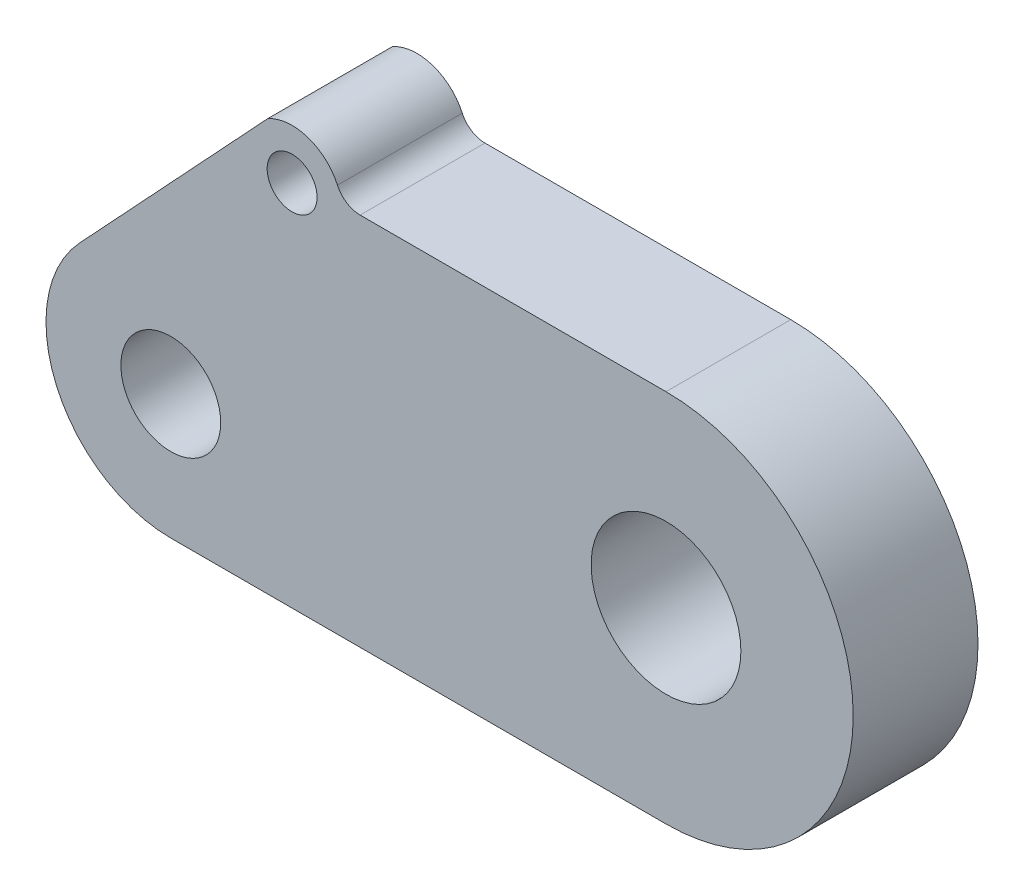
from build123d import *

# Parameters (mm, degrees)
SKETCH1_R           = 3
SKETCH1_R_2         = 1
SKETCH1_R_3         = 2
BOSS_EXTRUDE1_DEPTH = 5


with BuildPart() as part:
    # Sketch1 → Boss-Extrude1 (new body)
    with BuildSketch(Plane.XY):
        with BuildLine():
            Line((-19.84, -7.5), (0, -7.5))
            ThreePointArc((0, -7.5), (7.5, 0), (0, 7.5))
            Line((0, 7.5), (-12.252821971, 7.5))
            ThreePointArc((-12.252821971, 7.5), (-12.792883696, 7.658374588), (-13.161881314, 8.083333333))
            ThreePointArc((-13.161881314, 8.083333333), (-14.360041425, 9.15148662), (-15.957538412, 8.994826253))
            Line((-15.957538412, 8.994826253), (-23.496768508, 0.9099918))
            ThreePointArc((-23.496768508, 0.9099918), (-24.425300372, -4.493745345), (-19.84, -7.5))
        make_face()
        Circle(SKETCH1_R, mode=Mode.SUBTRACT)
        with Locations((-14.98, 7.25)):
            Circle(SKETCH1_R_2, mode=Mode.SUBTRACT)
        with Locations((-19.84, -2.5)):
            Circle(SKETCH1_R_3, mode=Mode.SUBTRACT)
    extrude(amount=BOSS_EXTRUDE1_DEPTH)


solid = part.part
